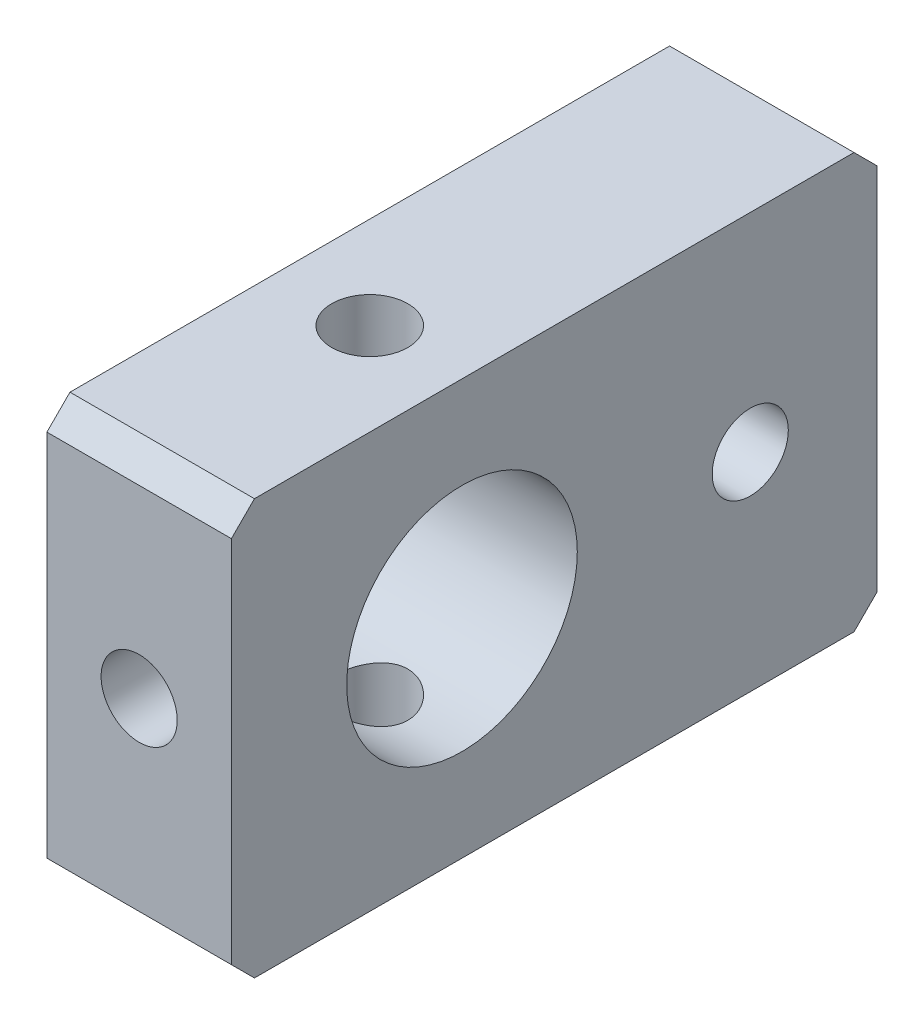
SolidWorks part; units mm, degrees
material "SUS304"
ref_plane "前视基准面" through (0, 0, 0) normal (0, 0, 1) x (1, 0, 0)
ref_plane "上视基准面" through (0, 0, 0) normal (0, 1, 0) x (1, 0, 0)
ref_plane "右视基准面" through (0, 0, 0) normal (1, 0, 0) x (0, 0, -1)
sketch "草图1" plane through (0, 0, 0) normal (1, 0, 0) x (0, 0, -1)
  line L1 (14, -9) -> (-14, -9)
  line L2 (14, -9) -> (14, 9)
  line L3 (14, 9) -> (-14, 9)
  line L4 (-14, -9) -> (-14, 9)
  line L5 (14, -9) -> (-14, 9) construction
  line L6 (14, 9) -> (-14, -9) construction
  point P0 (0, 0)
  dimension "D1" = 28
  dimension "D2" = 18
extrude "凸台-拉伸1" add sketch "草图1" along normal mid plane 8
sketch "草图2" plane through (4, 0, 0) normal (1, 0, 0) x (0, 0, -1)
  line L0 (-14, 0) -> (-4, 0) construction
  line L1 (-14, 9) -> (-14, -9) construction
  circle A0 centre (-4, 0) radius 5
  dimension "D1" = 10
  dimension "D2" = 10
extrude "切除-拉伸1" cut sketch "草图2" against normal through all
hole_wizard "M4 螺纹孔1" positions "草图6" profile "草图4" tap size "M4" standard "GB"
sketch "草图6" plane through (0, 0, 14) normal (0, 0, 1) x (1, 0, 0)
  point P0 (0, 0)
sketch "草图4" plane through (0, 0, 14) normal (1, 0, 0) x (0, -1, 0)
  line L0 (0, 0) -> (0, 5)
  line L1 (0, 5) -> (1.65, 5)
  line L2 (1.65, 5) -> (1.65, 0)
  line L5 (1.65, 0) -> (0, 0)
  line L11 (0, -6.35) -> (0, 107.95) construction
  dimension "通孔螺纹孔钻头直径" = 3.3
  dimension "通孔螺纹孔钻头深度" = 5
cosmetic thread "孔螺蚊线5"
hole_wizard "M4 螺纹孔2" positions "草图8" profile "草图9" tap size "M4" standard "GB" end condition through all
sketch "草图8" plane through (4, 0, 0) normal (1, 0, 0) x (0, 0, -1)
  line L0 (-4, 0) -> (8.5, 0) construction
  point P0 (8.5, 0)
  dimension "D1" = 12.5
sketch "草图9" plane through (4, 0, -8.5) normal (0, 1, 0) x (0, 0, -1)
  line L0 (0, 0) -> (0, 8)
  line L1 (0, 8) -> (1.65, 8)
  line L2 (1.65, 8) -> (1.65, 0)
  line L5 (1.65, 0) -> (0, 0)
  line L11 (0, -6.35) -> (0, 107.95) construction
  dimension "通孔螺纹孔钻头直径" = 3.3
  dimension "通孔螺纹孔钻头深度" = 8
cosmetic thread "孔螺蚊线9"
hole_wizard "M4 螺纹孔3" positions "草图10" profile "草图11" tap size "M4" standard "GB" end condition through all
sketch "草图10" plane through (0, 9, 0) normal (0, 1, 0) x (1, 0, 0)
  line L0 (4, 1) -> (4, -9) construction
  line L1 (4, 14) -> (4, -14) construction
  line L6 (-4, -4) -> (4, -4) construction
  line L8 (-4, 14) -> (-4, -14) construction
  point P0 (0, -4)
sketch "草图11" plane through (0, 9, 4) normal (1, 0, 0) x (0, 0, 1)
  line L0 (0, 0) -> (0, 18)
  line L1 (0, 18) -> (1.65, 18)
  line L2 (1.65, 18) -> (1.65, 0)
  line L5 (1.65, 0) -> (0, 0)
  line L11 (0, -6.35) -> (0, 107.95) construction
  dimension "通孔螺纹孔钻头直径" = 3.3
  dimension "通孔螺纹孔钻头深度" = 18
cosmetic thread "孔螺蚊线7"
chamfer "倒角1" distance 1 angle 45 4 edges at (0, -9, -14) (0, 9, -14) (0, -9, 14) (0, 9, 14)
